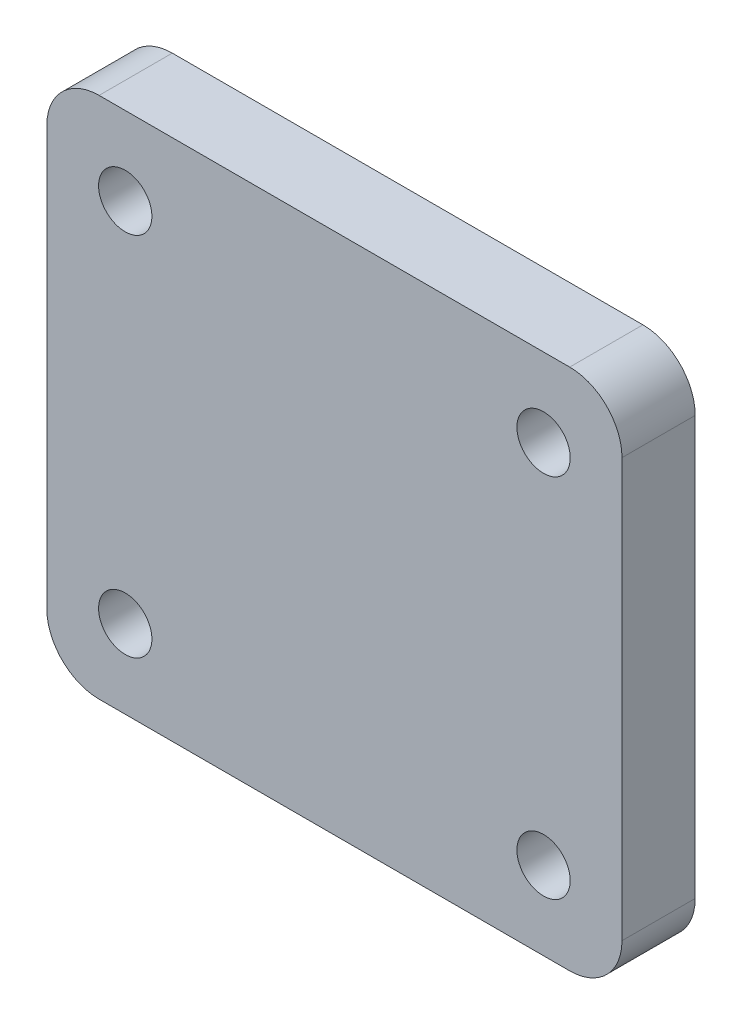
SolidWorks part; units mm, degrees
material "普通碳钢"
ref_plane "前视基准面" through (0, 0, 0) normal (0, 0, 1) x (1, 0, 0)
ref_plane "上视基准面" through (0, 0, 0) normal (0, 1, 0) x (1, 0, 0)
ref_plane "右视基准面" through (0, 0, 0) normal (1, 0, 0) x (0, 0, -1)
sketch "草图1" plane through (0, 0, 0) normal (0, 0, 1) x (1, 0, 0)
  line L1 (10, 0) -> (100, 0)
  line L2 (0, 10) -> (0, 90)
  line L3 (10, 100) -> (100, 100)
  line L4 (110, 10) -> (110, 90)
  arc A0 (10, 0) -> (0, 10) centre (10, 10) cw
  arc A1 (100, 0) -> (110, 10) centre (100, 10) ccw
  arc A2 (100, 100) -> (110, 90) centre (100, 90) cw
  arc A3 (0, 90) -> (10, 100) centre (10, 90) cw
  point P7 (0, 0)
  point P10 (110, 0)
  point P15 (0, 100)
  dimension "D3" = 10
  dimension "D1" = 100
  dimension "D2" = 110
extrude "凸台-拉伸1" add sketch "草图1" along normal blind 14
hole_wizard "M12 螺纹孔1" positions "3D草图1" profile "草图2" tap size "M12" standard "GB"
sketch3d "3D草图1"
  line L0 (15, 85, 14) -> (95, 85, 14) construction
  line L1 (95, 85, 14) -> (95, 15, 14) construction
  line L2 (95, 15, 14) -> (15, 15, 14) construction
  line L3 (15, 15, 14) -> (15, 85, 14) construction
  line L5 (0, 90, 14) -> (0, 10, 14) construction
  line L6 (100, 100, 14) -> (10, 100, 14) construction
  point P0 (15, 85, 14)
  point P2 (95, 85, 14)
  point P4 (95, 15, 14)
  point P6 (15, 15, 14)
  dimension "D1" = 80
  dimension "D2" = 70
  dimension "D3" = 15
  dimension "D4" = 15
sketch "草图2" plane through (15, 85, 14) normal (1, 0, 0) x (0, -1, 0)
  line L0 (0, 0) -> (0, 32.3144)
  line L1 (0, 32.3144) -> (5.1, 29.25)
  line L2 (5.1, 29.25) -> (5.1, 0)
  line L5 (5.1, 0) -> (0, 0)
  line L10 (0, 32.3144) -> (-5.1, 29.25) construction
  line L11 (0, -6.35) -> (0, 107.95) construction
  dimension "螺纹孔钻头直径" = 10.2
  dimension "螺纹孔钻头深度" = 29.25
  dimension "导头角度" = 118
cosmetic thread "孔螺蚊线1" parameters "D1"=14, "D2"=12
cosmetic thread "孔螺蚊线2" parameters "D1"=14, "D2"=12
cosmetic thread "孔螺蚊线3" parameters "D1"=14, "D2"=12
cosmetic thread "孔螺蚊线4" parameters "D1"=14, "D2"=12
